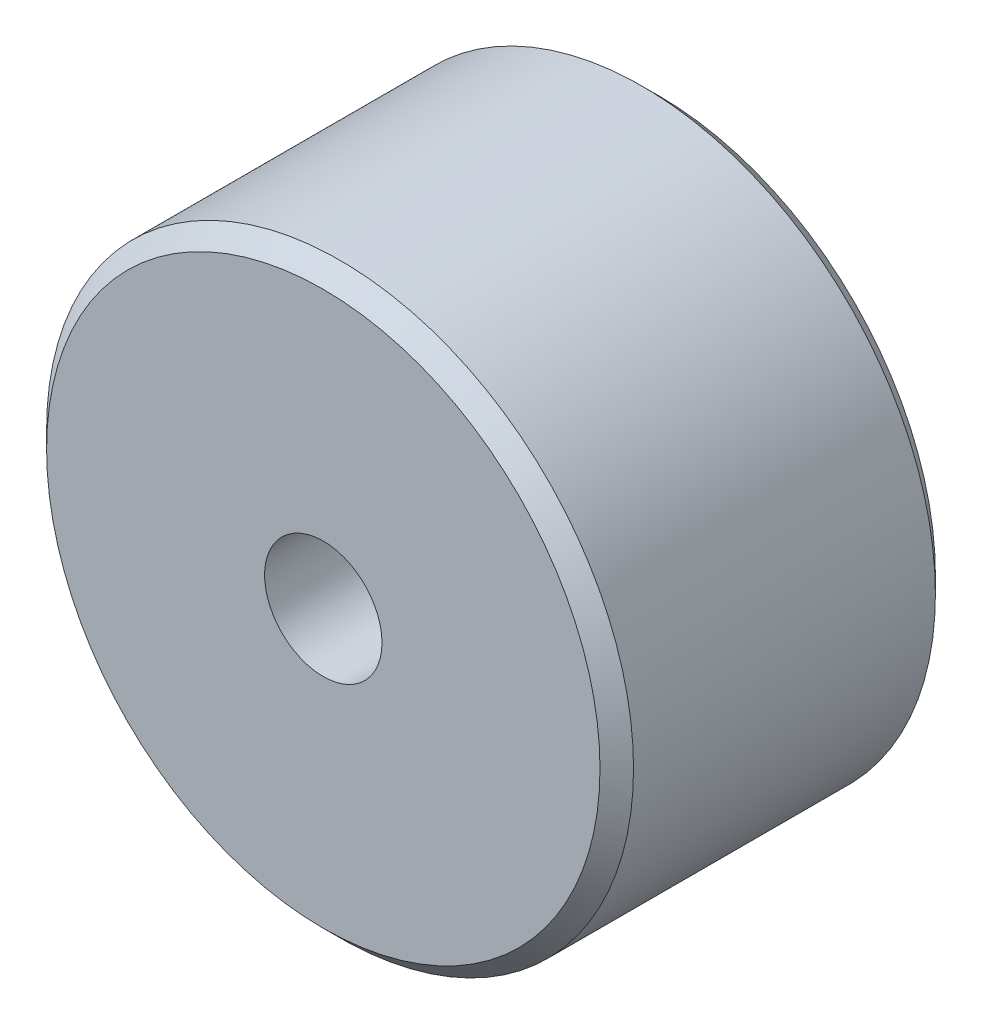
from build123d import *

# Parameters (mm, degrees)
SKETCH1_R           = 35
BOSS_EXTRUDE1_DEPTH = 40
CHAMFER1_SIZE       = 2
M16_TAPPED_HOLE1_D  = 14


with BuildPart() as part:
    # Sketch1 → Boss-Extrude1 (new body)
    with BuildSketch(Plane.XY):
        Circle(SKETCH1_R)
    extrude(amount=BOSS_EXTRUDE1_DEPTH)

    # Chamfer1
    chamfer1_edges = [part.edges().sort_by_distance(p)[0] for p in [
        (-35, 0, 0),
        (-35, 0, 40),
    ]]
    chamfer(chamfer1_edges, length=CHAMFER1_SIZE)

    # M16 Tapped Hole1 (through all)
    with Locations(Plane.XY.offset(40)):
        with Locations((0, 0)):
            Hole(M16_TAPPED_HOLE1_D / 2)


solid = part.part
